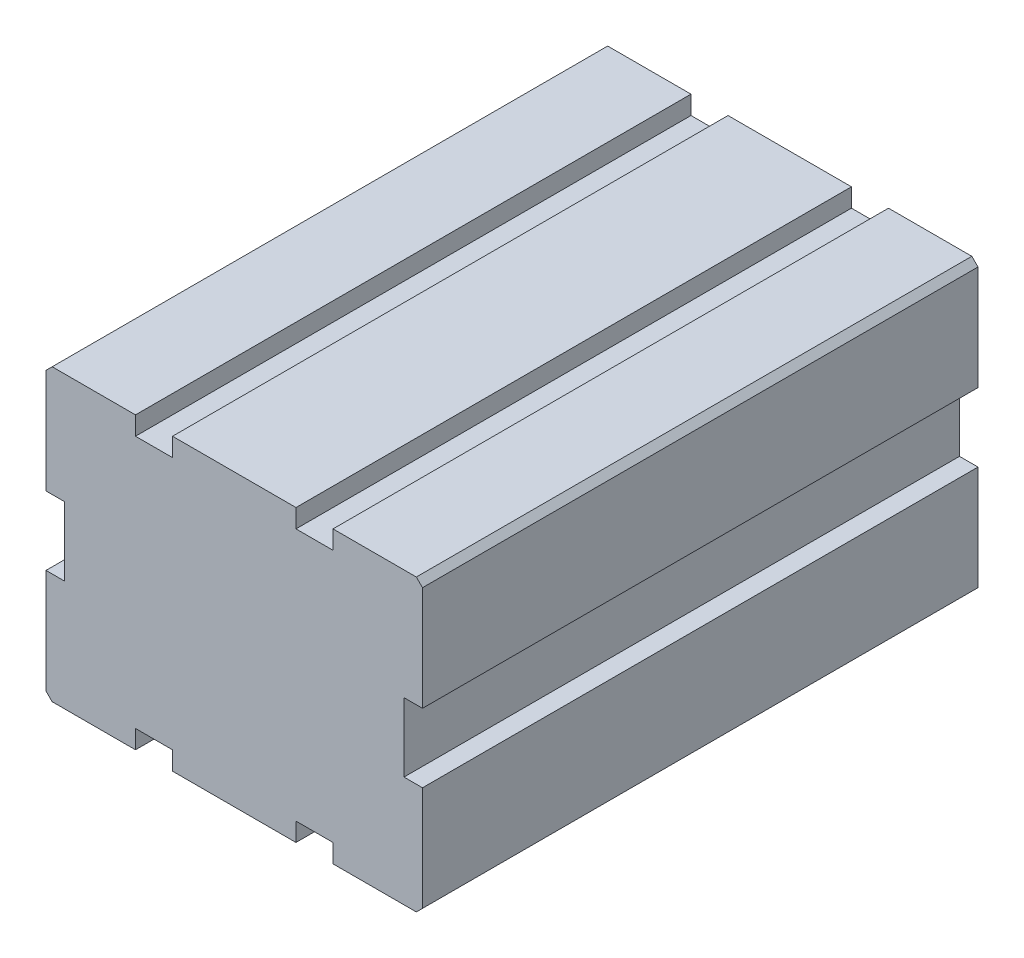
from build123d import *

# Parameters (mm, degrees)
BOSS_EXTRUDE2_DEPTH = 45


with BuildPart() as part:
    # Sketch1 → Boss-Extrude2 (new body)
    with BuildSketch(Plane.XY):
        Polygon((-15.25, 11.25), (-14.75, 11.75), (-8, 11.75), (-8, 10.25), (-5, 10.25), (-5, 11.75), (5, 11.75), (5, 10.25), (8, 10.25), (8, 11.75), (14.75, 11.75), (15.25, 11.25), (15.25, 2.78649269), (13.75, 2.78649269), (13.75, -2.78649269), (15.25, -2.78649269), (15.25, -11.25), (14.75, -11.75), (8, -11.75), (8, -10.25), (5, -10.25), (5, -11.75), (-5, -11.75), (-5, -10.25), (-8, -10.25), (-8, -11.75), (-14.75, -11.75), (-15.25, -11.25), (-15.25, -2.78649269), (-13.75, -2.78649269), (-13.75, 2.78649269), (-15.25, 2.78649269), align=None)
    extrude(amount=BOSS_EXTRUDE2_DEPTH)


solid = part.part
